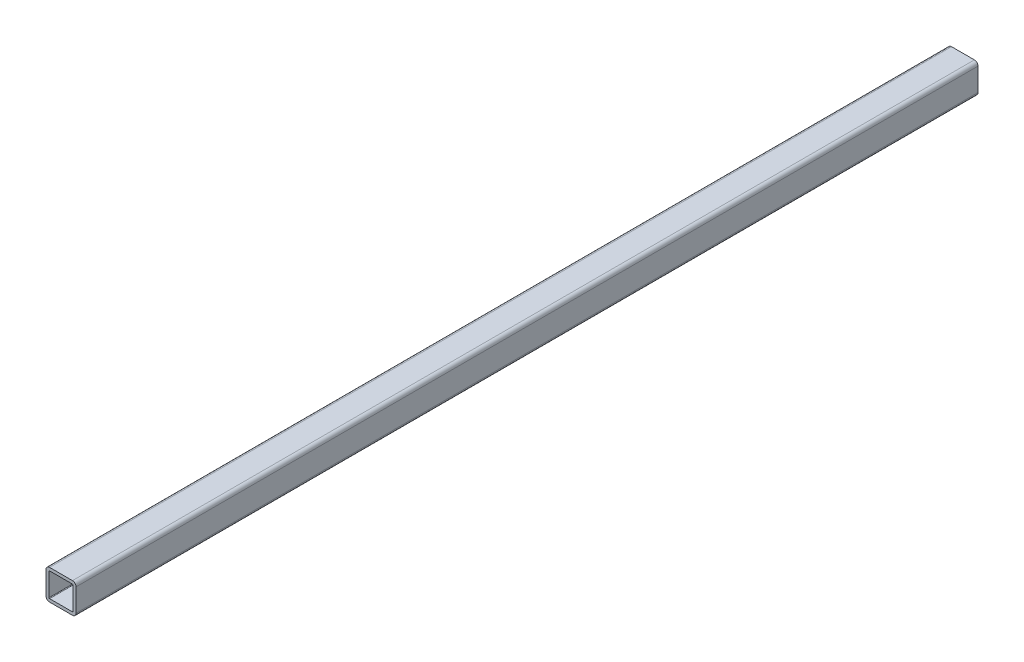
from build123d import *

# Parameters (mm, degrees)
BOSS_EXTRUDE1_DEPTH = 1500


with BuildPart() as part:
    # Sketch1 → Boss-Extrude1 (new body)
    with BuildSketch(Plane.XY):
        with BuildLine():
            Line((6, 0), (44, 0))
            ThreePointArc((44, 0), (48.242640687, 1.757359313), (50, 6))
            Line((50, 6), (50, 44))
            ThreePointArc((50, 44), (48.242640687, 48.242640687), (44, 50))
            Line((44, 50), (6, 50))
            ThreePointArc((6, 50), (1.757359313, 48.242640687), (0, 44))
            Line((0, 44), (0, 6))
            ThreePointArc((0, 6), (1.757359313, 1.757359313), (6, 0))
        make_face()
        with BuildLine():
            Line((6, 45), (44, 45))
            ThreePointArc((44, 45), (44.707106781, 44.707106781), (45, 44))
            Line((45, 44), (45, 6))
            ThreePointArc((45, 6), (44.707106781, 5.292893219), (44, 5))
            Line((44, 5), (6, 5))
            ThreePointArc((6, 5), (5.292893219, 5.292893219), (5, 6))
            Line((5, 6), (5, 44))
            ThreePointArc((5, 44), (5.292893219, 44.707106781), (6, 45))
        make_face(mode=Mode.SUBTRACT)
    extrude(amount=BOSS_EXTRUDE1_DEPTH)


solid = part.part
